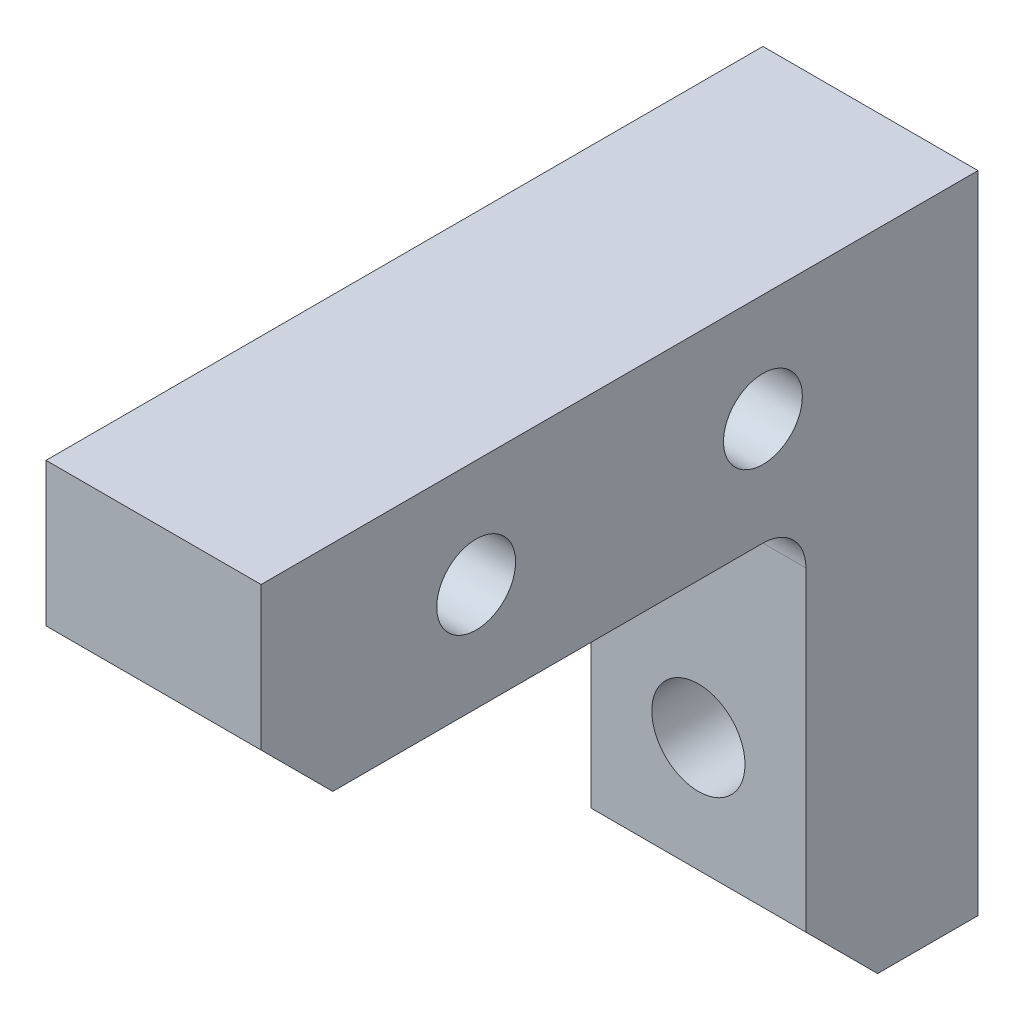
SolidWorks part; units mm, degrees
material "6061"
ref_plane "前视基准面" through (0, 0, 0) normal (0, 0, 1) x (1, 0, 0)
ref_plane "上视基准面" through (0, 0, 0) normal (0, 1, 0) x (1, 0, 0)
ref_plane "右视基准面" through (0, 0, 0) normal (1, 0, 0) x (0, 0, -1)
sketch "草图1" plane through (0, 0, 0) normal (0, 0, 1) x (1, 0, 0)
  line L1 (-7.5, -7.5) -> (7.5, -7.5)
  line L2 (-7.5, -7.5) -> (-7.5, 7.5)
  line L3 (-7.5, 7.5) -> (7.5, 7.5)
  line L4 (7.5, -7.5) -> (7.5, 7.5)
  line L5 (-7.5, -7.5) -> (7.5, 7.5) construction
  line L6 (-7.5, 7.5) -> (7.5, -7.5) construction
  point P0 (0, 0)
  dimension "D1" = 15
  dimension "D2" = 15
extrude "凸台-拉伸1" add sketch "草图1" along normal mid plane 50
sketch "草图2" plane through (0, 0, -25) normal (0, 0, -1) x (-1, 0, 0)
  line L0 (-7.5, -7.5) -> (-7.5, 7.5) construction
  line L1 (7.5, -7.5) -> (-7.5, -7.5)
  line L2 (7.5, -7.5) -> (7.5, -37.5)
  line L3 (7.5, -37.5) -> (-7.5, -37.5)
  line L4 (-7.5, -7.5) -> (-7.5, -37.5)
  dimension "D1" = 30
extrude "凸台-拉伸2" add sketch "草图2" against normal blind 12
hole_wizard "Ø6.5 (6.5) 直径孔1" positions "草图4" profile "草图3" hole size "Ø6.5" standard "ISO" end condition through all
sketch "草图4" plane through (0, 0, -13) normal (0, 0, 1) x (1, 0, 0)
  line L0 (7.5, -37.5) -> (-7.5, -37.5) construction
  point P0 (0, -24.5)
  dimension "D1" = 13
sketch "草图3" plane through (0, -24.5, -13) normal (1, 0, 0) x (0, -1, 0)
  line L0 (0, 0) -> (0, 12)
  line L1 (0, 12) -> (3.25, 12)
  line L2 (3.25, 12) -> (3.25, 0)
  line L5 (3.25, 0) -> (0, 0)
  line L11 (0, -6.35) -> (0, 107.95) construction
  dimension "通孔孔直径" = 6.5
  dimension "通孔孔深度" = 12
fillet "圆角1" radius 3 1 edges
chamfer "倒角2" distance 5 angle 45 2 edges at (0, -37.5, -13) (0, -7.5, 25)
hole_wizard "Ø5.5 (5.5) 直径孔1" positions "草图6" profile "草图5" hole size "Ø5.5" standard "GB" end condition through all
sketch "草图6" plane through (7.5, 0, 0) normal (1, 0, 0) x (0, 0, -1)
  line L3 (26.8318, 0) -> (-31.8024, 0) construction
  line L5 (-25, 7.5) -> (25, 7.5) construction
  line L6 (25, 7.5) -> (25, -37.5) construction
  point P0 (10, 0)
  point P2 (-10, 0)
  dimension "D1" = 7.5
  dimension "D2" = 15
  dimension "D3" = 20
sketch "草图5" plane through (7.5, 0, -10) normal (0, 1, 0) x (0, 0, -1)
  line L0 (0, 0) -> (0, 15)
  line L1 (0, 15) -> (2.75, 15)
  line L2 (2.75, 15) -> (2.75, 0)
  line L5 (2.75, 0) -> (0, 0)
  line L11 (0, -6.35) -> (0, 107.95) construction
  dimension "通孔孔直径" = 5.5
  dimension "通孔孔深度" = 15
